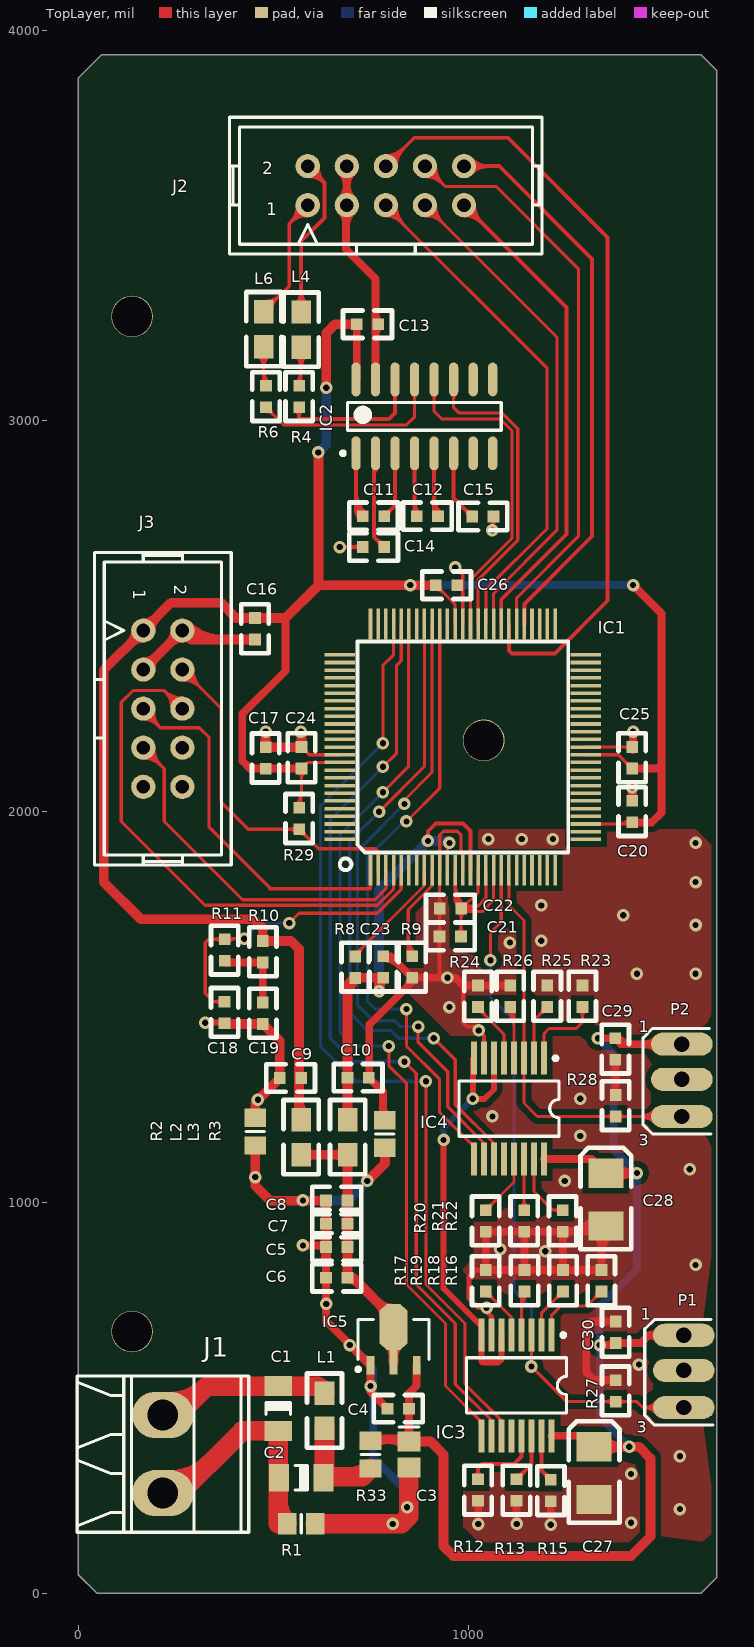
[diagram p0: TopLayer view]
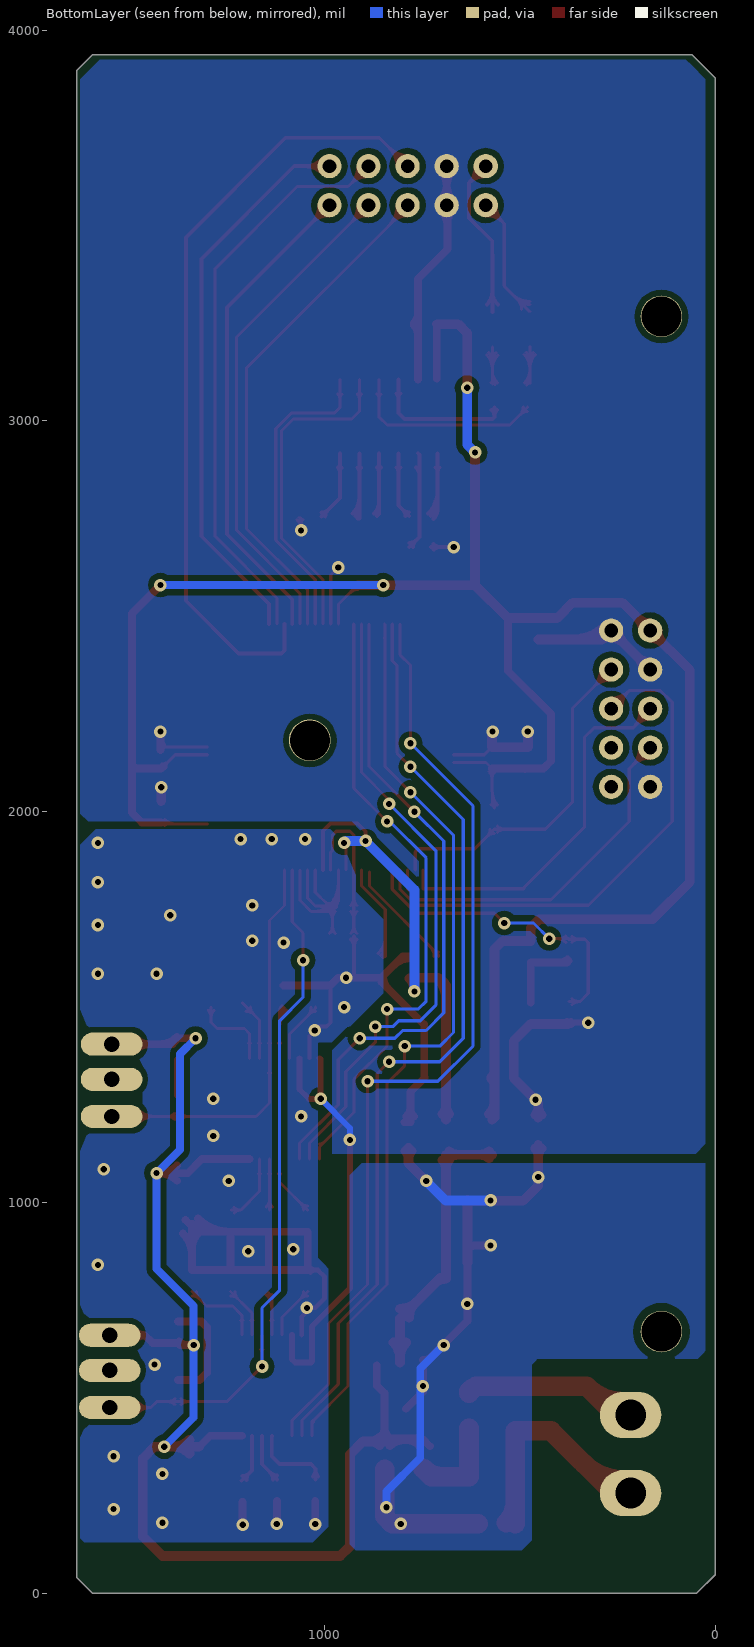
[diagram p1: BottomLayer view, seen from below]
# Altium PCB MISC67359.PcbDoc
Units mil, origin at the board's own origin, x right, y up, seen from the top; angles counter-clockwise.
Board outline 1633.86 x 3937.01 mil, 2 copper layers (TopLayer, BottomLayer); 72 components, 87 nets, 307 pads, 79 vias.

## Layer stack, top to bottom (the 12.6 mil dielectric is the usual default, probably not edited)
TopLayer: signal copper 1.4
Dielectric: core 12.6, FR-4, Dk 4.8
BottomLayer: signal copper 1.4

## Board outline
47.25,0 0,47.24 0,3877.95 59.06,3937.01 1594.49,3937.01 1633.86,3897.64 1633.86,39.37 1594.49,0

## Design rules (kind name [scope] priority, off if disabled: settings)
Clearance Clearance_1 [All vs InNet('DGND_MCU')] p1: gap=15
Clearance [All] p2: gap=8
DiffPairsRouting [All] p1: maxlimit=7 minlimit=7 mostfreqgap=7 maxuncoupledlength=500
FabricationTestPointUsage TestPointUsage [All] p1: valid=0 allowmultiple=FALSE
FabricationTestpoint Testpoint [All] p1: side=3 testpointundercomponent=TRUE minsize=40 maxsize=100 preferedsize=60 minholesize=20 maxholesize=40 preferedholesize=32 testpointgrid=1 allowsidetop=TRUE allowsidebottom=TRUE usegrid=TRUE gridtolerance=0.01
PlaneClearance [All] p1: clearance=10
PlaneConnect [All] p1: planeconnectstyle=Direct reliefexpansion=20 reliefentries=4 reliefconductorwidth=10 reliefairgap=10
PolygonConnect [All] p1: connectstyle=Direct reliefconductorwidth=12 reliefentries=4 polygonreliefangle="90 Angle"
RoutingLayers [All] p1: top layer_v5=FALSE bottom layer_v5=FALSE
RoutingVias [All] p1: holewidth=10 width=20 viastyle="Through Hole" minholewidth=10 minwidth=20 maxholewidth=28 maxwidth=50
SilkscreenOverComponentPads [All] p1: minsilkscreentomaskgap=10
SolderMaskExpansion [All] p1: expansion=4
Width width [All] p1: maxlimit=200 minlimit=7 preferedwidth=8
21 further rules are at their usual default settings.

## Components (designator, comment, footprint, x,y, rotation, side; value= is the part's Value field where it differs from the comment)
C1 "" CAPC3216N 511.81,472.44 r270 top (schematic designator C158)
C2 "" CAPC3216N 570.87,295.28 r180 top (schematic designator C158)
C3 "10u" CAPC2012N 846.46,354.33 r270 top (schematic designator C158)
C4 "0.1U" 0603 846.46,472.44 r180 top (schematic designator C158)
C5 "100n/50V" 0603 688.87,886.23 r180 top (schematic designator C158)
C6 "10n/50V" 0603 688.87,807.49 r180 top (schematic designator C158)
C7 "0.1U" 0603 634.08,945.28 r0 top (schematic designator C158)
C8 "0.1U" 0603 634.08,1004.34 r0 top (schematic designator C158)
C9 "0.1U" 0603 570.87,1318.9 r180 top (schematic designator C158)
C10 "0.1U" 0603 688.98,1318.9 r0 top (schematic designator C158)
C11 "100n/50V" 0603 728.35,2755.91 r0 top (schematic designator C158)
C12 "100n/50V" 0603 866.14,2755.91 r0 top (schematic designator C158)
C13 "100n/50V" 0603 767.72,3248.03 r180 top (schematic designator C158)
C14 "100n/50V" 0603 728.35,2677.17 r0 top (schematic designator C158)
C15 "100n/50V" 0603 1062.99,2755.91 r180 top (schematic designator C158)
C16 "0.1U" 0603 452.76,2440.94 r90 top (schematic designator C158)
C17 "0.1U" 0603 480,2110 r90 top (schematic designator C158)
C18 "1U" 0603 375.01,1458.85 r90 top (schematic designator C158)
C19 "0.1U" 0603 472.84,1456.8 r90 top (schematic designator C158)
C20 "0.1U" 0603 1417.32,2027.56 r270 top (schematic designator C158)
C21 "0.1U" 0603 925,1680 r0 top (schematic designator C158)
C22 "4.7U" 0603 925.2,1751.97 r0 top (schematic designator C158)
C23 "0.1U" 0603 780.2,1629.8 r270 top (schematic designator C158)
C24 "0.1U" 0603 570.87,2165.35 r270 top (schematic designator C158)
C25 "0.1U" 0603 1417.32,2165.35 r270 top (schematic designator C158)
C26 "0.1U" 0603 970,2580 r180 top (schematic designator C158)
C27 "22u" 3528 1320,375 r90 top
C28 "22u" 3528 1350,1075 r90 top
C29 "1U" 0603 1375,1365 r90 top (schematic designator C158)
C30 "1U" 0603 1375,695 r270 top (schematic designator C158)
IC1 "C8051F040" TQFP100 984.25,2165.35 r0 top
IC2 "MAX3232" SOIC127P600-16N 885.83,3011.81 r90 top (schematic designator J2)
IC3 "74HC-HCT4051" SOIC16 1122.05,531.5 r180 top
IC4 "74HC-HCT4051" SOIC16 1102.36,1240.16 r180 top
IC5 "AS117" SOT89L 807.09,649.61 r90 top
J1 "" MKDS3_2RMI 216.54,255.91 r90 top
J2 "" FKV10SN 787.4,3602.36 r0 top
J3 "" FKV10SN 216.54,2263.78 r270 top
L1 "1UH" 0805 629.92,511.81 r270 top (schematic designator C3)
L2 "1UH" 0805 570.87,1122.05 r90 top (schematic designator C3)
L3 "1UH" 0805 688.98,1211.84 r270 top (schematic designator C3)
L4 "600Ω/500mA-0805" 0805 570.87,3188.98 r90 top (schematic designator C3)
L6 "600Ω/500mA-0805" 0805 475,3190 r90 top (schematic designator C3)
P1 "" E3 1545,570 r0 top (schematic designator P2)
P2 "" E3 1540,1315 r0 top
R1 "0R" 6-0805_N 570.87,177.17 r0 top
R2 "0R" 6-0805_N 452.76,1181.1 r90 top
R3 "0R" 6-0805_N 785,1175 r90 top
R4 "100" 0603 565,3090 r270 top (schematic designator C158)
R6 "100" 0603 480,3090 r270 top (schematic designator C158)
R8 "0R" 0603 709.06,1574.7 r90 top (schematic designator C158)
R9 "0R" 0603 855,1575 r90 top (schematic designator C158)
R10 "10K" 0603 472.84,1614.28 r90 top (schematic designator C158)
R11 "1K" 0603 375.22,1618.54 r90 top (schematic designator C158)
R12 "10M 1%" 0603 1023.62,236.22 r90 top (schematic designator C158)
R13 "1M 1%" 0603 1122.05,236.22 r90 top (schematic designator C158)
R15 "100k 1%" 0603 1210,235 r90 top (schematic designator C158)
R16 "10k 1%" 0603 1338.58,826.77 r270 top (schematic designator C158)
R17 "1k 1%" 0603 1043.31,771.98 r90 top (schematic designator C158)
R18 "200R 1%" 0603 1240.16,826.77 r270 top (schematic designator C158)
R19 "100R 1%" 0603 1141.73,826.77 r270 top (schematic designator C158)
R20 "10M 1%" 0603 1043.31,925.2 r90 top (schematic designator C158)
R21 "1M 1%" 0603 1141.73,925.2 r90 top (schematic designator C158)
R22 "100k 1%" 0603 1240.16,925.2 r90 top (schematic designator C158)
R23 "10k 1%" 0603 1290,1555 r270 top (schematic designator C158)
R24 "1k 1%" 0603 1023.62,1500.32 r90 top (schematic designator C158)
R25 "200R 1%" 0603 1200,1555 r270 top (schematic designator C158)
R26 "100R 1%" 0603 1105,1555 r270 top (schematic designator C158)
R27 "100M 1%" 0603 1375,545 r270 top (schematic designator C158)
R28 "100M 1%" 0603 1375,1275 r270 top (schematic designator C158)
R29 "4.7K" 0603 565,2010 r270 top (schematic designator C158)
R33 "0R" 6-0805_N 748.03,354.33 r90 top

## Footprints (in the part's own frame and the unit in brackets; to place one, negate y for a bottom-side part, rotate by r counter-clockwise, add the part's x,y. Pads: shape width x height; smd on the part's side, far side on the other; paste and mask are expansions set on the pad)
6-0805_N [mm] "Chip Resistor, Body 2.0x1.2mm, IPC Medium Density"
  rect 1.2x1.4 smd: 1(-0.9,0) 2(0.9,0)
  silkscreen extent 0,-0.6 0,0.6, body extent -1.07,-0.7 1.07,0.7, height 0.7
0603 [mil]
  rect 30x30 smd: 1(-0.1,0.4) 2(54.9,0.4)
  silkscreen extent -35,-35 90,35
0805 [mil]
  rect 60x50 smd: 1(-0.1,0.38) 2(89.9,0.38)
  silkscreen extent -50,-45 140,45
3528 [mil]
  rect 75x90 smd: 1(-0.28,-0.48) 2(-135.28,-0.48)
  silkscreen extent -195,-65 65,65
CAPC2012N [mm] "Chip Capacitor, Body 2.0x1.3mm, IPC Medium Density"
  rect 1.3x1.5 smd: 1(-0.85,0) 2(0.85,0)
  silkscreen extent -1.8,-0.65 -1.8,0.65, body extent -1.1,-0.72 1.1,0.72, height 1.1
CAPC3216N [mm] "Chip Capacitor, Body 3.2x1.6mm, IPC Medium Density"
  rect 1.3x1.8 smd: 1(-1.45,0) 2(1.45,0)
  silkscreen extent -0.4,-0.8 0.4,0.8, body extent -1.7,-0.9 1.7,0.9, height 1.35
E3 [mm] "TO, Flat Index; 3 In-Line, Axial Leads; Body Dia. 4.6mm; Lead Dia. 0.5 mm (max)"
  oval 4x1.5 hole 1: 1(0.127,2.286) 2(0.127,0) 3(0.127,-2.413)
  silkscreen extent -2.41,-3.56 2.03,3.3
FKV10SN [mil]
  round 62 hole 35: 1(-200,-50) 2(-200,50) 3(-100,-50) 4(-100,50) 5(0,-50) 6(0,50) 7(100,-50) 8(100,50) 9(200,-50) 10(200,50)
  silkscreen extent -400,-175 400,175
MKDS3_2RMI [mm]
  oval 3x4 hole 2: 1(0,0) 2(5.08,0)
  silkscreen extent -2.54,-5.59 7.62,5.59
SOIC16 [mm]
  rect 0.4x2.15 smd: 1(-2.275,-3.275) 2(-1.625,-3.275) 3(-0.975,-3.275) 4(-0.325,-3.275) 5(0.325,-3.275) 6(0.975,-3.275) 7(1.625,-3.275) 8(2.275,-3.275) 9(2.275,3.275) 10(1.625,3.275) 11(0.975,3.275) 12(0.325,3.275) 13(-0.325,3.275) 14(-0.975,3.275) 15(-1.625,3.275) 16(-2.275,3.275)
  silkscreen extent -3.25,-3.4 3.25,1.8
SOIC127P600-16N [mm] "SOIC, 16-Leads, Body 9.9x3.9mm, Pitch 1.27mm, IPC Medium Density"
  oval 2.2x0.6 smd: 1(-2.4,4.445) 2(-2.4,3.175) 3(-2.4,1.905) 4(-2.4,0.635) 5(-2.4,-0.635) 6(-2.4,-1.905) 7(-2.4,-3.175) 8(-2.4,-4.445) 9(2.4,-4.445) 10(2.4,-3.175) 11(2.4,-1.905) 12(2.4,-0.635) 13(2.4,0.635) 14(2.4,1.905) 15(2.4,3.175) 16(2.4,4.445)
  silkscreen extent -2.52,-5 0.9,5.42, body extent -2,-5 2,5, height 1.75
SOT89L [mm] "SOT89, 3-Leads, Body 4.5x2.4 mm, Pitch 1.5mm, Lead Span 4.1mm, IPC High Density"
  rect 1.2x0.5 smd: 1(-1.7,1.5) 3(-1.7,-1.5)
  rect 1.6x0.5 smd: 2(-1.5,0)
  oct 3x1.8 smd: 2(0.8,0)
  silkscreen extent -2.07,-2.3 1.3,2.42, body extent -1.3,-2.3 1.3,2.3, height 1.6
TQFP100 [mm]
  rect 0.23x2 smd: 1(-6,-8) 2(-5.5,-8) 3(-5,-8) 4(-4.5,-8) 5(-4,-8) 6(-3.5,-8) 7(-3,-8) 8(-2.5,-8) 9(-2,-8) 10(-1.5,-8) 11(-1,-8) 12(-0.5,-8) 13(0,-8) 14(0.5,-8) 15(1,-8) 16(1.5,-8) 17(2,-8) 18(2.5,-8) 19(3,-8) 20(3.5,-8) 21(4,-8) 22(4.5,-8) 23(5,-8) 24(5.5,-8) 25(6,-8) 51(6,8) 52(5.5,8) 53(5,8) 54(4.5,8) 55(4,8) 56(3.5,8) 57(3,8) 58(2.5,8) 59(2,8) 60(1.5,8) 61(1,8) 62(0.5,8) 63(0,8) 64(-0.5,8) 65(-1,8) 66(-1.5,8) 67(-2,8) 68(-2.5,8) 69(-3,8) 70(-3.5,8) 71(-4,8) 72(-4.5,8) 73(-5,8) 74(-5.5,8) 75(-6,8)
  rect 2x0.23 smd: 26(8,-6) 27(8,-5.5) 28(8,-5) 29(8,-4.5) 30(8,-4) 31(8,-3.5) 32(8,-3) 33(8,-2.5) 34(8,-2) 35(8,-1.5) 36(8,-1) 37(8,-0.5) 38(8,0) 39(8,0.5) 40(8,1) 41(8,1.5) 42(8,2) 43(8,2.5) 44(8,3) 45(8,3.5) 46(8,4) 47(8,4.5) 48(8,5) 49(8,5.5) 50(8,6) 76(-8,6) 77(-8,5.5) 78(-8,5) 79(-8,4.5) 80(-8,4) 81(-8,3.5) 82(-8,3) 83(-8,2.5) 84(-8,2) 85(-8,1.5) 86(-8,1) 87(-8,0.5) 88(-8,0) 89(-8,-0.5) 90(-8,-1) 91(-8,-1.5) 92(-8,-2) 93(-8,-2.5) 94(-8,-3) 95(-8,-3.5) 96(-8,-4) 97(-8,-4.5) 98(-8,-5) 99(-8,-5.5) 100(-8,-6)
  silkscreen extent -8,-8 6.86,6.86

## Part data
C1 C3: library part Cap2, "Capacitor"
C2: library part CAP, "Capacitor"
C4 C7 C8 C9 C10 C16 C17 C18 C19 C20 C21 C22 C23 C24 C25 C26 C29 C30: library part CAP, "Capacito"
C5 C6 C11 C12 C13 C14 C15: library part "CAPACITOR NON-PO"
C27 C28: library part "CAPACITOR POL"
IC1: library part C8051F020
IC3 IC4: library part CD54HC4051
IC5: library part "Volt Reg", "Voltage Regulator"
J1: library part "Header 2", "Header, 2-Pin"
J2 J3: library part "HEADER 5X2"
L1 L2 L3: library part INDUCTO
L4 L6: library part BEA
P1 P2: library part MHDR1X3
R1 R2 R3 R33: library part RES, "Resistor"
R4 R6: library part SMDRXX_
R8 R9: library part RES, "Resisto"
R10 R11 R12 R13 R15 R16 R17 R18 R19 R20 R21 R22 R23 R24 R25 R26 R27 R28 R29: library part RES

## Free pads (board coordinates)
  round 106.3 hole 102.36: 0(137.8,669.29) 0(137.8,3267.72) 0(1037.8,2182.72)

## Via types
v1: diameter 32, hole 16, TopLayer to BottomLayer, 79 vias

## Nets (pads, with @x,y where several pads share a name; then routed paths per layer and width w, separated by ;. In a path a pad name is that pad's centre, name@x,y a point inside that pad or via, vN(x,y) a via of type N, cw(c..) or ccw(c..) an arc to the next point about the centre after c; other vN are vias at no path point)
3.3VA_MCU: C10.1 C23.2 IC1.11 IC1.14 L3.1 R8.1 | length 1454.6
  TopLayer w8: IC1.11 944.88,1914.88 v1(950,1920)
  TopLayer w10: v1(895,1925) 895,1950 915,1970 985,1970 1003.94,1951.06 IC1.14
  TopLayer w25: L3.1@680.52,1225.78 ccw(c659.18,1247.12) 689.36,1247.12 ccw(c719.54,1247.12) L3.1@698.2,1225.78 ; L3.1 689.36,1555 709.17,1574.8 C23.2@770,1574.8 ; 689.36,1521.96 cw(c761.3,1521.96) R8.1@710.43,1572.83 ; 689.36,1547.09 cw(c715.12,1547.09) R8.1@709.23,1572.16 ; v1@770,1543.28 cw(c812.22,1543.28) C23.2@782.37,1573.14 ; C23.2@770,1574.31 v1(770,1540) v1@770.6,1540.6
  BottomLayer w25: v1@770.6,1540.6 770,1541.2 770,1800 v1(895,1925) 945,1925 v1(950,1920)
3.3VD_MCU: C9.1 C13.2 C16.2 C17.1 C20.2 C24.2 C25.2 C26.2 IC1.28 IC1.37 IC1.64 IC1.90 IC2.16 J3.1 L2.2 R10.2 R29.1 | length 6622.1
  TopLayer w8: C17.1 C24.2@564.6,2109.9 ; C17.1@487.38,2102.12 cw(c506.16,2083.34) 506.16,2109.9 cw(c506.16,2136.45) C17.1@487.38,2117.68 ; 543.36,2109.9 ccw(c543.36,2138.36) C24.2@563.49,2118.23 ; 546.06,2109.9 cw(c546.06,2085.25) 563.49,2102.68 cw(c544.71,2083.9) 571.27,2083.9 cw(c597.82,2083.9) C24.2@579.05,2102.68 ; R29.1@557.62,2017.88 ccw(c527.74,2047.76) 570,2047.76 ; R29.1@563.28,2012.22 ccw(c547.06,2028.45) 570,2028.45 ; R29.1 570,2014.7 570,2050 ; 570,2025.56 ccw(c580.86,2025.56) R29.1@573.18,2017.88 ; 571.27,2051.27 C24.2 586.8,2125.98 IC1.90 ; C26.2@915.1,2568.6 cw(c915.1,2541.32) 934.39,2560.61 ; C26.2 932.55,2562.15 ; C26.2@915.69,2568.61 cw(c916.87,2546.47) 932.55,2562.15 ; C26.2@915.77,2568.62 cw(c917.13,2546.43) 932.85,2562.15 ; C26.2@926.09,2579.01 ccw(c948.23,2577.83) 932.55,2562.15 ; C26.2@926.1,2579.24 ccw(c949.18,2578.48) 932.85,2562.15 ; C26.2@926.1,2579.6 ccw(c951.94,2579.6) 933.67,2561.33 ; IC1.64 964.57,2530.43 932.85,2562.15 ; IC1.28 C20.2@1413.57,1968.5 ; IC1.37 1382.51,2145.67 C25.2 ; 1381.13,1968.5 ccw(c1381.13,2009.25) C20.2@1409.95,1980.44 ; 1400.45,1968.5 ccw(c1400.45,1989.94) C20.2@1415.6,1974.78 ; 1401.2,1968.5 cw(c1401.2,1956.14) C20.2@1409.95,1964.88 ; C25.2@1406.72,2110.46 ccw(c1380.17,2110.46) 1398.95,2129.23 ccw(c1417.72,2148.01) C25.2@1417.72,2121.46 ; 932.55,2562.15 932.85,2562.15
  TopLayer w20: 530.84,2495.84 530.84,2360.84 420,2250 420,2130 439.54,2110.46 C24.2 ; IC2.16@712.82,3108.29 C13.2 ; C20.2 1467.66,1972.66 1492.66,1997.66 1492.66,2120 ; C25.2 1483.12,2110.46 1492.66,2120 ; v1(1420,2580) 1492.66,2507.34 1492.66,2120
  TopLayer w25: J3.1@148.04,2463.78 cw(c103.37,2463.78) 134.95,2432.2 cw(c166.54,2400.62) J3.1@166.54,2445.28 ; J3.1@166.54,2482.28 ccw(c166.54,2526.94) 198.12,2495.36 ccw(c229.7,2463.78) J3.1@185.04,2463.78 ; 565,1260.36 ccw(c613.9,1260.36) L2.2@579.32,1225.78 ; 565,1298.05 cw(c591.41,1298.05) C9.1@572.74,1316.73 ; 565,1338.94 ccw(c591.41,1338.94) C9.1@572.74,1320.26 ; L2.2 565,1217.43 565,1648.35 544.17,1669.17 R10.2 472.44,1702.56 450,1725 160,1725 65,1820 65,2362.24 J3.1 237.76,2535 365,2535 404.16,2495.84 C16.2 530.84,2495.84 614.6,2579.6 ; v1(614.6,2919.6) 614.6,2579.6 ; v1(635,3085) 635,3225 657.63,3247.63 C13.2 ; C26.2 614.6,2579.6
  BottomLayer w20: v1(850,2580) v1(1420,2580)
  BottomLayer w25: v1(614.6,2919.6) 635,2940 v1(635,3085)
3V3: C5.1 C6.1 C7.2 C8.2 IC5.2 L2.1 L3.2 | length 1054.1
  TopLayer w25: L2.1 688.59,1121.95 688.98,1121.56 C8.2 C7.2 C5.1 C6.1 702.91,807.09 807.09,702.91 807.09,681.1 IC5.2@807.09,590.55 ; L2.1@579.32,1113.11 cw(c600.66,1091.77) 600.66,1121.95 cw(c600.66,1152.12) L2.1@579.32,1130.78 ; L3.2@680.52,1108.11 cw(c660.1,1087.69) 688.98,1087.69 ; L3.2@680.52,1113.11 ccw(c659.18,1091.77) 659.18,1121.95 ccw(c659.18,1152.12) L3.2@680.52,1130.78 ; C6.1@688.98,804.59 cw(c688.98,764.9) 717.04,792.96 ; 688.98,1085.85 cw(c720.46,1085.85) L3.2@698.2,1108.11 ; 764.85,745.15 ccw(c807.09,787.4) IC5.2@807.09,727.66 ; 769.22,740.78 cw(c733.16,704.72) IC5.2@784.15,704.72 ; IC5.2@790.87,641.26 cw(c751.72,602.12) 807.09,602.12 cw(c862.45,602.12) IC5.2@823.3,641.26
+5V: C3.1 C4.1 C27.1 C28.1 C29.2 C30.2 IC3.16 IC4.16 IC5.3 P1.1 P2.1 R33.2 | length 4106.7
  TopLayer w20: R33.2@730.42,376.09 R33.2@748.03,393.7 ; C3.1@835.43,398.82 ccw(c808.82,425.43) 846.46,425.43 ccw(c884.1,425.43) C3.1@857.48,398.82 ; C3.1@846.46,388.09 846.46,511.81 866.14,531.5 IC5.3 ; IC4.16 1313.98,1111.22 C28.1 1429.72,1074.72 v1(1430,1075) ; IC3.16 1292.64,402.56 C27.1 ; v1(1330,1420) 1374.5,1420 C29.2 1389.5,1405 P2.1 ; v1(1335,635) 1370.3,635 C30.2 1440.1,640.1 1460,660 ; 1351.01,635 ccw(c1351.01,664.49) C30.2@1371.87,643.64 ; C28.1@1377.43,1055.27 cw(c1424.37,1008.32) 1424.37,1074.72 cw(c1424.37,1141.11) C28.1@1377.43,1094.16 ; C29.2@1378.13,1423.43 ccw(c1422.64,1467.93) 1422.64,1405 ; P2.1@1481.98,1391.19 ccw(c1448.64,1357.86) 1448.64,1405 ccw(c1448.64,1452.14) P2.1@1481.98,1418.81 ; P1.1@1485.58,647.76 ccw(c1460,627.17) 1460,660 ; P1.1@1485.58,672.24 cw(c1460,692.83) 1460,660 ; P1.1 1460,660
  TopLayer w25: R33.2@759.83,381.9 cw(c788.32,353.41) 788.32,393.7 ; R33.2@767.72,393.7 C3.1@828.94,393.7 ; 796.66,393.7 cw(c796.66,341.93) C3.1@833.26,378.54 ; C3.1 902.2,387.8 935,355 935,120 960,95 1415,95 1465,145 1465,345 1435.28,374.72 C27.1 ; C3.1@859.65,378.54 cw(c882,356.19) 882,387.8 cw(c882,419.4) C3.1@859.65,397.05 ; C27.1@1345.66,357.04 cw(c1388.34,314.36) 1388.34,374.72 cw(c1388.34,435.07) C27.1@1345.66,392.39
  BottomLayer w20: v1(1330,1420) 1370,1380 1370,1135 v1(1430,1075) 1430,830 1335,735 v1(1335,635) 1335,449.72 v1(1410,374.72)
/RD: IC1.92
/WR: IC1.91
A0: IC1.80
A1: IC1.79
A1N0.0: IC1.18 IC3.3 P1.3 R27.2 | length 2077.4
  TopLayer w8: v1(1055,1620) 1055,1690 1082.68,1717.68 IC1.18 ; IC3.3@1157.69,623.24 cw(c1151.08,616.63) 1160.43,616.63 cw(c1169.79,616.63) IC3.3@1163.17,623.24 ; v1(1160,580) v1@1160.43,579.57 ; IC3.3 v1@1160.43,579.57 ; R27.2@1367.62,482.32 ccw(c1348.84,463.55) 1348.84,490.1 ccw(c1348.84,516.66) R27.2@1367.62,497.88 ; R27.2@1383.18,482.32 cw(c1401.96,463.55) 1401.96,490.1 cw(c1401.96,516.66) R27.2@1383.18,497.88 ; P1.3@1481.47,458.31 ccw(c1445,426.81) 1445,475 ; P1.3@1481.47,491.69 cw(c1445,523.19) 1445,475 ; P1.3@1487.52,463.54 ccw(c1462.48,441.91) 1462.48,475 ccw(c1462.48,508.09) P1.3@1487.52,486.46 ; P1.3 1445,475 ; v1@1160.43,579.57 1249.9,490.1 R27.2 1429.9,490.1 1445,475
  BottomLayer w8: v1(1055,1620) 1055,1525 1115,1465 1115,775 1160,730 v1(1160,580)
A1N0.1: IC1.19 IC4.3 P2.3 R28.2 | length 1306.6
  TopLayer w8: IC1.19 1102.36,1760 1140.75,1721.61 IC4.3 1140.75,1254.25 1175,1220 P2.3 ; IC4.3@1138.01,1331.91 cw(c1131.4,1325.29) 1140.75,1325.29 cw(c1150.1,1325.29) IC4.3@1143.49,1331.91 ; IC4.3@1138.01,1406.28 ccw(c1131.4,1412.9) 1140.75,1412.9 ccw(c1150.1,1412.9) IC4.3@1143.49,1406.28 ; 1348.6,1220 ccw(c1348.6,1246.91) R28.2@1367.62,1227.88 ; 1349.09,1220 cw(c1349.09,1193.79) R28.2@1367.62,1212.32 ; R28.2@1383.18,1212.32 cw(c1401.71,1193.79) 1401.71,1220 ; R28.2@1383.18,1227.88 ccw(c1402.2,1246.91) 1402.2,1220 ; P2.3@1477.74,1201.95 ccw(c1434.16,1158.37) 1434.16,1220 ccw(c1434.16,1281.63) P2.3@1477.74,1238.05 ; P2.3@1483.39,1207.61 ccw(c1453.47,1177.68) 1453.47,1220 ccw(c1453.47,1262.32) P2.3@1483.39,1232.39
A2: IC1.78
A3: IC1.77
A4: IC1.76
A5: IC1.75
A6: IC1.74
A7: IC1.73
A8: IC1.88
A9: IC1.87
A10: IC1.86
A11: IC1.85
A12: IC1.84
A13: IC1.83
AGND_MCU: C10.2 C21.1 C22.1 C23.1 C27.2 C28.2 C29.1 C30.1 IC1.10 IC1.13 IC3.7 IC4.7 R3.2 R9.1 R12.1 R13.1 R15.1 R16.1 R17.2 R18.1 R19.1 R20.1 R21.1 R22.1 R23.1 R24.2 R25.1 R26.1 R27.1 R28.1 | length 3903.8
  TopLayer w8: C21.1@917.12,1688.18 ccw(c897.87,1707.43) 925.09,1707.43 ; C22.1@917.32,1744.59 cw(c898.54,1725.81) 925.09,1725.81 cw(c951.65,1725.81) C22.1@932.87,1744.59 ; C22.1@917.32,1760.15 ccw(c898.54,1778.93) 925.09,1778.93 ccw(c951.65,1778.93) C22.1@932.87,1760.15 ; C21.1@925.09,1693.31 C22.1 925.09,1850.29 IC1.10 925.2,1940.2 935,1950 970,1950 980,1940 980,1900 985,1895 985,1851.14 IC1.13 ; 925.09,1706.48 ccw(c950.98,1706.48) C21.1@932.68,1688.18
  TopLayer w10: C21.1@917.83,1673.33 cw(c900.76,1656.26) 924.9,1656.26 cw(c949.04,1656.26) C21.1@931.97,1673.33 ; 924.9,1575.1 C21.1 ; 985.22,1555.22 985.22,1459.78 995,1450 1015,1450 1038.39,1426.61 IC4.7 ; R12.1 R12.1@1023.62,235.72
  TopLayer w12: R17.2@1036.54,820.51 ccw(c1021.18,805.15) 1021.18,826.87 ccw(c1021.18,848.6) R17.2@1036.54,833.24 ; R17.2 1016.87,826.87 1000,810 1000,754.29 1024.29,730 1035,730 1058.07,706.93 IC3.7
  TopLayer w20: R3.2@771.43,1220.07 ccw(c750.74,1240.75) 780,1240.75 ; 780,1245.89 ccw(c816.52,1245.89) R3.2@790.7,1220.07 ; C23.1@780.6,1624.91 cw(c780.6,1566.98) 821.56,1607.94 ; C23.1 799.59,1629.91 R9.1@854.5,1575 ; R3.2@795.55,1205 780,1205 780,1283.17 C10.2 745,1320.42 745,1455 854.5,1564.5 R9.1@854.5,1575 ; 838.78,1548.78 ccw(c812.66,1574.9) R9.1@849.6,1574.9 ; R9.1 R9.1@854.5,1575 ; v1@1023.62,177.17 R12.1@1023.62,235.72 ; R26.1@1105.28,1555.22 R24.2 985.22,1555.22 965.44,1575 R9.1@854.5,1575 ; v1@1121.65,177.57 R13.1 ; R21.1@1142.13,924.29 R19.1 ; v1(1209.6,175) R15.1@1209.6,233.95 ; R22.1@1240.56,924.29 R18.1 ; R22.1@1241.29,925.09 ccw(c1241.29,1041.4) C28.2@1323.54,959.16 ; 1289.58,925.09 ccw(c1289.58,993.12) C28.2@1337.68,945.02 ; C28.2@1323.54,920.27 cw(c1286.24,882.98) 1338.98,882.98 ; 1338.98,863.67 cw(c1419.02,863.67) C28.2@1362.43,920.27 ; C28.2@1355.48,954.72 C28.2@1338.98,938.22 ; C29.1 1375.4,1364.1 R28.1 ; R27.1 1319.9,545.1 1300,565 1300,680 1315.1,695.1 C30.1 ; R19.1 R18.1 ; R19.1 R17.2 R20.1 R21.1 R22.1 1325.86,925.09 C28.2@1338.98,938.22 ; R18.1 R16.1 C28.2@1338.98,938.22
  other v1: 1024.02,176.76 1122.05,177.17 1415,180 1540,215 1415,305 1540,350 1435,585 1045,730 1580,840 1195,875 1080,880 1245,1055 1565,1085 1285,1170 1060,1220 1285,1265 1025,1440 950,1500 945,1575 1430,1585 1580,1585 1105,1665 1185,1670 1580,1710 1395,1735 1185,1760 1580,1820 1580,1920 1050,1930 1135,1930 1215,1930
D0: IC1.72 IC3.11 | length 2452.7
  TopLayer w8: v1(780,2175) 780,2375 807.09,2402.09 IC1.72 ; v1(890,1310) 890,790 990,690 990,535 1083.66,441.34 IC3.11
  BottomLayer w8: v1(780,2175) 620,2015 620,1400 710,1310 v1(890,1310)
D1: IC1.71 IC3.10 | length 2400.3
  TopLayer w8: v1(780,2115) 815,2150 815,2375 826.77,2386.77 IC1.71 ; v1(835,1360) 865,1330 865,790 965,690 965,535 1058.07,441.93 IC3.10
  BottomLayer w8: v1(780,2115) 645,1980 645,1420 705,1360 v1(835,1360)
D2: IC1.70 IC3.9 | length 2373.3
  TopLayer w8: v1(780,2050) 845,2115 845,2478.86 IC1.70 ; v1(795,1400) 795,1350 840,1305 840,790 940,690 940,530 1032.48,437.52 IC3.9 ; 845,2440.68 cw(c851.25,2440.68) IC1.70@846.83,2445.1 ; IC3.9@1025.5,444.5 cw(c1018.02,437.01) IC3.9@1028.61,437.01 ; IC3.9@1026.74,443.26 ccw(c1032.48,449) IC3.9@1032.48,440.88
  BottomLayer w8: v1(780,2050) 670,1940 670,1435 705,1400 v1(795,1400)
D3: IC1.69
D4: IC1.68 IC4.11 | length 1688.8
  TopLayer w8: v1(770,2000) 885.83,2115.83 IC1.68 ; v1(910,1420) 965,1365 965,1250 1063.98,1151.02 IC4.11
  BottomLayer w8: v1(770,2000) 695,1925 695,1485 740,1440 800,1440 820,1420 v1(910,1420)
D5: IC1.67 IC4.10 | length 1640.5
  TopLayer w8: v1(835,2020) 835,2030 905.51,2100.51 IC1.67 ; v1(870,1450) 870,1410 945.59,1334.41 945.59,1244.41 1038.39,1151.61 IC4.10
  BottomLayer w8: v1(835,2020) 715,1900 715,1505 755,1465 810,1465 825,1450 v1(870,1450)
D6: IC1.66 IC4.9 | length 1633.6
  TopLayer w8: v1(840,1495) 840,1400 925,1315 925,1230 1012.8,1142.2 IC4.9 ; v1(840,1975) 925.2,2060.2 IC1.66 ; 1000.27,1154.73 ccw(c1012.8,1167.26) IC4.9@1012.8,1149.54
  BottomLayer w8: v1(840,1975) 833.18,1975 740,1881.82 740,1515 760,1495 v1@850,1495
D7: IC1.65
DAC0: IC1.100
DGND_MCU: C9.2 C13.1 C14.1 C15.1 C16.1 C17.2 C18.1 C19.1 C20.1 C24.1 C25.1 C26.1 IC1.38 IC1.63 IC1.89 IC2.15 IC3.6 IC3.8 IC4.6 IC4.8 J2.3 J2.4 J3.2 J3.3 J3.9 R2.2 | length 4031.4
  TopLayer w8: C24.1 591.05,2145.67 IC1.89 ; J2.3@685,3549.96 J2.3 ; v1(965,2625) 984.25,2605.75 IC1.63 ; C15.1@1055.32,2747.73 cw(c1044.01,2736.42) 1060,2736.42 ; v1@1060,2710 v1(1060,2720) C15.1@1060,2751.4 ; v1@1060,2721.48 cw(c1097.12,2721.48) C15.1@1070.87,2747.73 ; C15.1@1060,2740.79 cw(c1077.81,2740.79) C15.1@1065.22,2753.38 ; IC1.38 C25.1@1417.62,2165.35
  TopLayer w10: v1@669.29,2677.57 C14.1 ; C14.1@721.17,2670.5 ccw(c704.1,2653.42) 704.1,2677.57 ccw(c704.1,2701.71) C14.1@721.17,2684.64
  TopLayer w15: v1(325,1460) 396.69,1460 ; 353.48,1460 cw(c353.48,1437.62) C18.1@369.3,1453.44 ; 359.52,1460 ccw(c359.52,1473.83) C18.1@369.3,1464.05 ; C18.1@379.91,1453.44 cw(c395.73,1437.62) 395.73,1460 ; C18.1@379.91,1464.05 ccw(c389.69,1473.83) 389.69,1460 ; v1(935,1160) 935,780 1032.48,682.52 IC3.8 1032.48,592.52 1035,590 1075,590 1083.66,598.66 IC3.6 ; IC4.8 1010,1366.3 v1(1010,1265) 1040,1265 1063.98,1288.98 IC4.6
  TopLayer w20: J2.3@672.55,3537.51 cw(c642.5,3507.46) 685,3507.46 ; J2.3@672.55,3567.21 ccw(c636.7,3603.06) 687.4,3603.06 ccw(c738.1,3603.06) J2.3@702.25,3567.21 ; J2.4@672.55,3637.51 cw(c636.7,3601.66) 687.4,3601.66 cw(c738.1,3601.66) J2.4@702.25,3637.51 ; 685,3495.87 cw(c743.9,3495.87) J2.3@702.25,3537.51 ; J2.3@685,3549.96 685,3440 760.83,3364.17 IC2.15 ; J2.3 J2.4 ; 760.83,3218.68 cw(c796.77,3218.68) C13.1@771.35,3244.09 ; 760.83,3276.58 ccw(c796.77,3276.58) C13.1@771.35,3251.17 ; C25.1@1414.19,2168.99 ccw(c1400.16,2183.02) 1420,2183.02 ; C25.1@1420,2158.18 v1(1420,2205)
  TopLayer w25: J3.3 J3.2 289.47,2440.84 ; J3.3@166.54,2382.28 ccw(c166.54,2426.94) 198.12,2395.36 ccw(c229.7,2363.78) J3.3@185.04,2363.78 ; J3.2@248.04,2463.78 cw(c203.37,2463.78) 234.95,2432.2 cw(c266.54,2400.62) J3.2@266.54,2445.28 ; J3.2@261.94,2459.18 ccw(c306.22,2503.46) 306.22,2440.84 ; J3.2@271.13,2445.86 cw(c275.9,2427.28) 289.47,2440.84 ; J3.2@279.62,2476.86 ccw(c366.57,2563.82) 366.57,2440.84 ; J3.2@284.45,2459.18 ccw(c303.04,2454.41) 289.47,2440.84 ; C18.1 376.66,1456.69 C19.1 515.97,1413.17 C9.2 v1(460,1262.53) 452.76,1255.28 R2.2 ; R2.2@444.89,1224.4 ccw(c425.9,1243.39) 452.76,1243.39 ccw(c479.61,1243.39) R2.2@460.62,1224.4 ; C16.1 289.47,2440.84 ; v1@479.6,2194.6 C17.2 C24.1@570.71,2164.9 ; C24.1 v1@571.27,2196.27 ; C20.1 v1(1417.72,2062.72)
  BottomLayer w8: v1@955,2625 v1(965,2625)
  BottomLayer w15: v1(935,1160) 935,1190 v1(1010,1265)
  other v1: 480,2205 570,2205 669.29,2677.17
GND: C3.2 C4.2 C5.2 C6.2 C7.1 C8.1 IC5.1 R1.2 R2.1 R3.1 | length 2224.4
  TopLayer w20: v1(575,890) 629.8,890 C5.2 ; 611.83,890 cw(c611.83,863.68) C5.2@630.44,882.29 ; 633.98,845 C6.2 633.98,696.73 IC5.1 v1(748.03,530) 748.03,515.57 C4.2 ; 724.78,605.93 ccw(c748.03,629.19) IC5.1@748.03,596.3
  TopLayer w25: R2.1@444.89,1137.8 cw(c425.9,1118.82) 452.76,1118.82 cw(c479.61,1118.82) R2.1@460.62,1137.8 ; R2.1@452.76,1146.59 v1(452.76,1065) 452.76,1043.31 492.13,1003.94 C8.1@633.98,1003.94 ; 633.98,845 C5.2 C7.1 C8.1@633.98,1003.94 ; C8.1 C8.1@633.98,1003.94 ; C8.1@634.78,1003.94 C8.1@633.98,1003.94 ; v1(740,1055) 785,1100 R3.1 ; R3.1@777.14,1131.7 cw(c758.15,1112.72) 785,1112.72 cw(c811.85,1112.72) R3.1@792.86,1131.7
  TopLayer w50: R1.2 v1(805,177.17) 826.77,177.17 846.46,196.85 C3.2@846.46,317.2
  BottomLayer w20: v1(695,635) 755,575 755,346.46 841.46,260 v1(841.46,220)
  BottomLayer w25: v1(575,1005) 690,1005 v1(740,1055)
  other v1: 635,740
HARD_RESET: IC1.53
NetC1_1: C1.1 J1.2 L1.1 | length 587.3
  TopLayer w50: J1.2 255.91,455.91 329.53,529.53 C1.1 612.69,529.53 L1.1 ; J1.2@236.22,489.96 ccw(c236.22,619.7) 327.96,527.96 ; 599.85,529.53 cw(c599.85,486.46) L1.1@630.3,516.91
NetC1_2: C1.2 C2.2 J1.1 R1.1 | length 805
  TopLayer w20: R1.1@511.81,200.79 R1.1
  TopLayer w50: J1.1 260.91,255.91 420.35,415.35 C1.2 511.81,200.79 R1.1@511.81,177.17 ; J1.1@236.22,289.96 ccw(c236.22,431.77) 336.5,331.5 ; 511.81,234.8 ccw(c589.14,234.8) R1.1@534.46,180.13
NetC2_1: C2.1 L1.2 R33.1 | length 305.3
  TopLayer w50: L1.2 630.3,297.63 726.76,297.63 R33.1 ; 696.07,297.63 ccw(c696.07,366.93) R33.1@745.07,317.92
NetC11_1: C11.1 IC2.1 | length 372.1
  TopLayer w10: IC2.1@706.01,2881.01 cw(c694.38,2869.38) 710.83,2869.38 cw(c727.27,2869.38) IC2.1@715.64,2881.01 ; 710.83,2774.21 ccw(c746.15,2774.21) C11.1@721.17,2749.24 ; 710.83,2798.36 ccw(c770.29,2798.36) C11.1 710.83,2773.72 IC2.1 ; 710.83,2822.5 ccw(c794.44,2822.5) C11.1@735.32,2763.38 ; C11.1@718.24,2756.31 ccw(c694.1,2756.31) 711.17,2773.38 ccw(c728.24,2790.45) C11.1@728.24,2766.31
NetC11_2: C11.2 IC2.3 | length 236.2
  TopLayer w10: C11.2 810.83,2783.89 IC2.3 ; C11.2@783.24,2766.31 ccw(c783.24,2790.45) 800.32,2773.38 ccw(c817.39,2756.31) C11.2@793.24,2756.31 ; IC2.3@806.01,2881.01 cw(c794.38,2869.38) 810.83,2869.38 cw(c827.27,2869.38) IC2.3@815.64,2881.01
NetC12_1: C12.1 IC2.4 | length 221.9
  TopLayer w10: IC2.4@856.01,2881.01 cw(c844.38,2869.38) 860.83,2869.38 cw(c877.27,2869.38) IC2.4@865.64,2881.01 ; 860.83,2793.03 ccw(c902.77,2793.03) C12.1@873.11,2763.38 ; IC2.4 860.83,2761.52 C12.1
NetC12_2: C12.2 IC2.5 | length 270.8
  TopLayer w10: IC2.5@906.01,2881.01 cw(c894.38,2869.38) 910.83,2869.38 cw(c927.27,2869.38) IC2.5@915.64,2881.01 ; 910.83,2780.96 ccw(c945.69,2780.96) C12.2 ; 910.83,2805.1 ccw(c969.84,2805.1) C12.2@928.11,2763.38 ; IC2.5 910.83,2750.59 C12.2@915.32,2750.59
NetC14_2: C14.2 IC2.2 | length 312.5
  TopLayer w10: 757.24,2860.73 cw(c785.92,2860.73) IC2.2@765.64,2881.01 ; IC2.2 757.24,2913.74 757.24,2703.57 C14.2 ; C14.2@773.24,2677.57 ccw(c749.1,2677.57) 766.17,2694.64 ccw(c783.24,2711.71) C14.2@783.24,2687.57
NetC15_2: C15.2 IC2.6 | length 245.1
  TopLayer w10: IC2.6@956.01,2881.01 cw(c944.38,2869.38) 960.83,2869.38 cw(c977.27,2869.38) IC2.6@965.64,2881.01 ; IC2.6 960.83,2802.77 C15.2 ; C15.2@998.09,2755.5 ccw(c973.95,2755.5) 991.02,2772.58 ccw(c1008.09,2789.65) C15.2@1008.09,2765.5
NetC18_2: C18.2 IC1.5 R11.2 | length 920.6
  TopLayer w8: C18.2@366.83,1505.97 ccw(c348.05,1487.19) 348.05,1513.75 ccw(c348.05,1540.3) C18.2@366.83,1521.53 ; R11.2@367.04,1665.66 ccw(c348.26,1646.88) 348.26,1673.43 ccw(c348.26,1699.99) R11.2@367.04,1681.21 ; C18.2 346.25,1513.75 325,1535 325,1665 333.43,1673.43 R11.2 376.38,1675 v1(425,1675) ; R11.2@382.6,1665.66 cw(c405.16,1643.09) 405.16,1675 ; R11.2@382.6,1681.21 ccw(c397.59,1696.21) 397.59,1675 ; v1(540,1715) 565,1740 765,1740 826.77,1801.77 IC1.5
  BottomLayer w8: v1(425,1675) 465,1715 v1(540,1715)
NetC19_2: C19.2 R10.1 R11.1 | length 222.8
  TopLayer w20: R11.1 379.08,1614.17 R10.1 C19.2 ; R11.1@378.35,1621.97 ccw(c397.17,1640.79) 397.17,1614.17
NetIC1_1: IC1.1 J3.5 | length 1141.7
  TopLayer w8: J3.5@166.54,2236.78 cw(c166.54,2184.43) 203.55,2221.45 ; J3.5@166.54,2244.78 cw(c166.54,2211.74) 189.9,2235.1 ; J3.5 166.54,2258.46 210,2215 ; J3.5@177.48,2262.73 ccw(c206.91,2259.89) 186.01,2238.99 ; J3.5@185.45,2261.96 ccw(c228.79,2257.79) 198,2227 ; J3.5@193.41,2261.19 ccw(c250.68,2255.68) 210,2215 ; IC1.1 748.03,1802.64 490,1802.64 490,1805 335,1960 335,2190 310,2215 210,2215
NetIC1_2: IC1.2 J3.4 R29.2 | length 1139.9
  TopLayer w8: J3.4@266.54,2336.78 cw(c266.54,2271.6) 312.63,2317.69 cw(c358.72,2363.78) J3.4@293.54,2363.78 ; J3.4@266.54,2344.78 cw(c266.54,2298.91) 298.97,2331.34 cw(c331.41,2363.78) J3.4@285.54,2363.78 ; J3.4 365,2265.31 365,2025 434.9,1955.1 R29.2 615.5,1905 760,1905 767.72,1897.28 IC1.2 ; R29.2@557.62,1947.32 ccw(c538.84,1928.55) 538.84,1955.1 ccw(c538.84,1981.66) R29.2@557.62,1962.88 ; R29.2@565.4,1944.1 cw(c565.4,1917.55) 584.18,1936.32 cw(c602.96,1955.1) R29.2@576.4,1955.1
NetIC1_3: IC1.3 J3.7 | length 1095.2
  TopLayer w8: J3.7@166.54,2136.78 cw(c166.54,2071.6) 212.63,2117.69 cw(c258.72,2163.78) J3.7@193.54,2163.78 ; J3.7@166.54,2144.78 cw(c166.54,2098.91) 198.97,2131.34 cw(c231.41,2163.78) J3.7@185.54,2163.78 ; J3.7 220,2110.31 220,1975 420.36,1774.64 759.63,1774.64 787.4,1802.41 IC1.3
NetIC1_4: IC1.4 J3.6 | length 1518.8
  TopLayer w8: J3.6@239.54,2263.78 ccw(c174.35,2263.78) 220.44,2309.87 ccw(c266.54,2355.96) J3.6@266.54,2290.78 ; J3.6@247.54,2263.78 ccw(c201.67,2263.78) 234.1,2296.21 ccw(c266.54,2328.65) J3.6@266.54,2282.78 ; J3.6 220.31,2310 140,2310 110,2280 110,1975 324.36,1760.64 765.43,1760.64 807.09,1802.3 IC1.4
NetIC1_8: IC1.8 R8.2 | length 330.4
  TopLayer w8: R8.2 708.66,1633.66 885,1810 IC1.8@885,1845.24 ; R8.2@708.66,1640.6 ccw(c708.66,1657.35) 720.5,1645.5 ; R8.2@719.66,1629.6 cw(c756.03,1629.6) 730.31,1655.31
NetIC1_9: IC1.9 R9.2 | length 343.2
  TopLayer w8: R9.2@844.6,1629.9 844.6,1749.6 905.51,1810.51 IC1.9 ; R9.2@844.6,1641.97 ccw(c866.67,1641.97) R9.2@851.06,1626.36 ; 844.6,1661.28 ccw(c885.98,1661.28) R9.2@856.72,1632.02 ; 844.6,1680.6 ccw(c905.3,1680.6) R9.2@862.38,1637.68
NetIC2_13: IC2.13 R6.2 | length 574.5
  TopLayer w8: R6.2@480.4,3024.1 cw(c480.4,2997.55) 499.18,3016.32 cw(c517.96,3035.1) R6.2@491.4,3035.1 ; R6.2 525.5,2990 840,2990 860.83,3010.83 IC2.13 ; IC2.13@855.3,3069.28 cw(c841.97,3055.95) 860.83,3055.95 cw(c879.68,3055.95) IC2.13@866.35,3069.28
NetIC2_14: IC2.14 R4.2 | length 428.6
  TopLayer w10: R4.2@558.33,3028.03 cw(c541.26,3010.96) 565.4,3010.96 cw(c589.54,3010.96) R4.2@572.47,3028.03 ; R4.2 565.4,3009.6 570,3005 795,3005 810.83,3020.83 IC2.14 ; IC2.14@806.01,3069.99 cw(c794.38,3058.36) 810.83,3058.36 cw(c827.27,3058.36) IC2.14@815.64,3069.99
NetIC3_1: IC3.1 R16.2 | length 259.9
  TopLayer w8: IC3.1@1208.87,697.62 ccw(c1202.26,704.23) 1211.61,704.23 ccw(c1220.97,704.23) IC3.1@1214.35,697.62 ; IC3.1 1211.61,711.61 1235,735 1302.11,735 R16.2 ; R16.2@1327.98,771.87 cw(c1301.43,771.87) 1320.21,753.1 cw(c1338.98,734.32) R16.2@1338.98,760.87
NetIC3_2: IC3.2 R18.2 | length 190.4
  TopLayer w8: IC3.2@1183.28,697.62 ccw(c1176.67,704.23) 1186.02,704.23 ccw(c1195.38,704.23) IC3.2@1188.76,697.62 ; IC3.2 1186.02,717.34 R18.2 ; R18.2@1229.56,771.87 cw(c1203,771.87) 1221.78,753.1 cw(c1240.56,734.32) R18.2@1240.56,760.87
NetIC3_4: IC3.4 R19.2 | length 184.5
  TopLayer w8: IC3.4@1132.1,697.62 ccw(c1125.49,704.23) 1134.84,704.23 ccw(c1144.19,704.23) IC3.4@1137.58,697.62 ; IC3.4 R19.2@1134.84,764.58 ; 1134.84,727.71 cw(c1186.29,727.71) R19.2@1149.91,764.1 ; 1134.84,747.03 cw(c1166.98,747.03) R19.2@1144.25,769.75
NetIC3_5: IC3.5 R17.1 | length 180.6
  TopLayer w8: R17.1@1042.91,760.87 cw(c1042.91,734.32) 1061.68,753.1 cw(c1080.46,771.87) R17.1@1053.91,771.87 ; R17.1 1109.25,705.53 IC3.5
NetIC3_13: IC3.13 R12.2 | length 242.6
  TopLayer w10: R12.2@1016.15,298.19 ccw(c999.08,315.26) 1023.22,315.26 ccw(c1047.36,315.26) R12.2@1030.29,298.19 ; R12.2 1023.22,318.22 1035,330 1115,330 1135,350 1135,402.4 IC3.13
NetIC3_14: IC3.14 R13.2 | length 165.4
  TopLayer w10: R13.2 1160.43,329.91 IC3.14 ; R13.2@1121.65,301.12 ccw(c1121.65,325.26) 1138.72,308.19 ccw(c1155.79,291.12) R13.2@1131.65,291.12
NetIC3_15: IC3.15 R15.2 | length 163.9
  TopLayer w10: IC3.15 1186.02,313.98 R15.2@1212.5,287.5 ; 1192.17,307.83 cw(c1174.24,289.9) R15.2@1199.6,289.9 ; 1193.39,306.61 ccw(c1209.6,322.82) R15.2@1209.6,299.9
NetIC4_1: IC4.1 R23.2 | length 269.2
  TopLayer w8: IC4.1@1189.19,1406.28 ccw(c1182.58,1412.9) 1191.93,1412.9 ccw(c1201.28,1412.9) IC4.1@1194.67,1406.28 ; IC4.1 1191.93,1431.93 1205,1445 1275,1445 1290.4,1460.4 R23.2 ; R23.2@1282.62,1492.32 cw(c1263.84,1473.55) 1290.4,1473.55 cw(c1316.96,1473.55) R23.2@1298.18,1492.32
NetIC4_2: IC4.2 R25.2 | length 216.2
  TopLayer w8: IC4.2@1163.6,1406.28 ccw(c1156.99,1412.9) 1166.34,1412.9 ccw(c1175.69,1412.9) IC4.2@1169.08,1406.28 ; IC4.2 1166.34,1466.34 R25.2@1210.55,1510.55 ; 1181.11,1481.11 cw(c1200.4,1461.82) R25.2@1200.4,1489.1 ; 1181.83,1481.83 ccw(c1163.57,1500.1) R25.2@1189.4,1500.1
NetIC4_4: IC4.4 R26.2 | length 245.3
  TopLayer w8: R26.2@1097.62,1492.32 cw(c1055.29,1449.99) 1115.16,1449.99 ; R26.2@1103.28,1497.98 cw(c1074.61,1469.31) 1115.16,1469.31 ; R26.2 1115.16,1490.35 IC4.4 ; R26.2@1108.94,1503.64 cw(c1093.92,1488.62) R26.2@1115.16,1488.62 ; IC4.4@1112.42,1406.28 ccw(c1105.8,1412.9) 1115.16,1412.9 ccw(c1124.51,1412.9) IC4.4@1117.9,1406.28
NetIC4_5: IC4.5 R24.1 | length 200.3
  TopLayer w8: R24.1@1023.22,1489.22 cw(c1023.22,1470.97) 1036.12,1483.88 ; R24.1 1023.22,1496.78 1089.57,1430.43 IC4.5 ; R24.1@1034.22,1500.22 ccw(c1069.09,1500.22) 1044.43,1475.57
NetIC4_13: IC4.13 R20.2 | length 217.5
  TopLayer w8: R20.2 1115.16,1052.35 IC4.13 ; R20.2@1042.91,991.09 ccw(c1042.91,1017.65) 1061.68,998.87 ccw(c1080.46,980.09) R20.2@1053.91,980.09 ; IC4.13@1112.42,1074.03 cw(c1105.8,1067.42) 1115.16,1067.42 cw(c1124.51,1067.42) IC4.13@1117.9,1074.03
NetIC4_14: IC4.14 R21.2 | length 187.8
  TopLayer w8: R21.2@1133.55,987.87 ccw(c1116.18,1005.24) 1140.75,1005.24 ; IC4.14@1138.01,1074.03 cw(c1131.4,1067.42) 1140.75,1067.42 cw(c1150.1,1067.42) IC4.14@1143.49,1074.03 ; 1140.75,1008.06 ccw(c1169.29,1008.06) R21.2@1149.11,987.87 ; IC4.14 1140.75,980.68 R21.2
NetIC4_15: IC4.15 R22.2 | length 228.4
  TopLayer w8: IC4.15@1163.6,1074.03 cw(c1156.99,1067.42) 1166.34,1067.42 cw(c1175.69,1067.42) IC4.15@1169.08,1074.03 ; IC4.15 1166.34,1028.66 1214.91,980.09 ; R22.2@1231.61,972.7 ccw(c1214.91,957.53) 1214.91,980.09 ; R22.2@1231.61,987.49 cw(c1214.91,1002.66) 1214.91,980.09 ; R22.2 1214.91,980.09
NetJ2_1: J2.1 L6.2 | length 607.4
  TopLayer w8: L6.2 540,3345.28 540,3504.96 J2.1 ; L6.2@474.62,3297.9 ccw(c474.62,3341.35) 505.35,3310.63 ; L6.2@474.62,3305.9 ccw(c474.62,3368.67) 519,3324.28 ; L6.2@495.62,3284.9 cw(c534.25,3284.9) 506.93,3312.21 ; J2.1@560.4,3552.36 cw(c495.22,3552.36) 541.31,3506.27 cw(c587.4,3460.18) J2.1@587.4,3525.36 ; J2.1@568.4,3552.36 cw(c522.53,3552.36) 554.97,3519.93 cw(c587.4,3487.49) J2.1@587.4,3533.36
NetJ2_2: J2.2 L4.2 | length 640.6
  TopLayer w10: L4.2@556.34,3298.02 ccw(c522.2,3332.16) 570.48,3332.16 ccw(c618.77,3332.16) L4.2@584.63,3298.02 ; L4.2 570.48,3424.82 570.87,3425.2 570.87,3460.43 629.92,3519.49 629.92,3609.84 ; J2.2 629.92,3609.84 ; J2.2@587.9,3636.37 cw(c588.97,3601.6) 613.57,3626.2 cw(c638.16,3650.8) J2.2@603.39,3651.87 ; J2.2@588.2,3626.37 cw(c589.95,3569.87) 629.92,3609.84 ; J2.2@613.39,3651.56 ccw(c669.89,3649.82) 629.92,3609.84
NetL4_1: L4.1 R4.1 | length 283.7
  TopLayer w8: L4.1@555.64,3169.03 cw(c519.79,3133.18) 570.48,3133.18 cw(c621.18,3133.18) L4.1@585.33,3169.03 ; R4.1@557.62,3097.88 ccw(c526.57,3128.93) 570.48,3128.93 ; L4.1@561.29,3174.68 cw(c539.1,3152.49) 570.48,3152.49 cw(c601.87,3152.49) L4.1@579.68,3174.68 ; R4.1@563.28,3092.22 ccw(c545.89,3109.62) 570.48,3109.62 ; R4.1@570.48,3095.19 L4.1 ; R4.1@570.48,3104.39 ccw(c579.69,3104.39) R4.1@573.18,3097.88
NetL6_1: L6.1 R6.1 | length 280.5
  TopLayer w8: L6.1@459.77,3170.05 cw(c423.92,3134.2) 474.62,3134.2 cw(c525.32,3134.2) L6.1@489.47,3170.05 ; L6.1@465.43,3175.71 cw(c443.23,3153.51) 474.62,3153.51 cw(c506,3153.51) L6.1@483.81,3175.71 ; R6.1@474.62,3095.89 L6.1 ; 474.62,3111.31 ccw(c501.61,3111.31) R6.1@482.52,3092.22 ; 474.62,3130.62 ccw(c520.92,3130.62) R6.1@488.18,3097.88
P0.2: IC1.60 J2.5 | length 1512.2
  TopLayer w8: J2.5@787.4,3525.36 cw(c787.4,3471.68) 825.36,3509.64 ; J2.5@787.4,3533.36 cw(c787.4,3498.99) 811.7,3523.3 ; J2.5 787.4,3547.6 1200,3135 1200,2725 1043.31,2568.31 IC1.60 ; J2.5@798.4,3552.36 ccw(c836.46,3552.36) 809.55,3525.45 ; J2.5@806.4,3552.36 ccw(c863.77,3552.36) 823.21,3511.79 ; J2.5@814.4,3552.36 ccw(c891.09,3552.36) 836.86,3498.14
P0.3: IC1.59 J2.7 | length 1453.6
  TopLayer w8: J2.7@887.4,3525.36 cw(c887.4,3459.61) 933.9,3506.1 ; J2.7@887.4,3533.36 cw(c887.4,3486.92) 920.24,3519.76 ; J2.7 887.64,3552.36 1225,3215 1225,2720 1062.99,2557.99 IC1.59 ; J2.7@906.4,3552.36 ccw(c951.7,3552.36) 919.67,3520.33 ; J2.7@914.4,3552.36 ccw(c979.02,3552.36) 933.33,3506.67
P0.4: IC1.58 J2.9 | length 1409.5
  TopLayer w10: J2.9@987.4,3526.36 cw(c987.4,3463.02) 1032.19,3507.81 ; J2.9@987.4,3536.36 cw(c987.4,3497.16) 1015.12,3524.88 ; J2.9 987.64,3552.36 1250,3290 1250,2710 1082.68,2542.68 IC1.58 ; J2.9@1003.4,3552.36 ccw(c1041.46,3552.36) 1014.55,3525.45 ; J2.9@1013.4,3552.36 ccw(c1075.6,3552.36) 1031.62,3508.38
P0.5: IC1.57 J2.6 | length 2172
  TopLayer w10: J2.6 860.04,3725 1100,3725 1355,3470 1355,2540 1220,2405 1110,2405 1102.36,2412.64 IC1.57 ; J2.6@787.4,3668.36 ccw(c787.4,3706.99) 814.72,3679.68 ccw(c842.03,3652.36) J2.6@803.4,3652.36 ; J2.6@787.4,3678.36 ccw(c787.4,3741.13) 831.79,3696.75 ccw(c876.17,3652.36) J2.6@813.4,3652.36
P0.6: IC1.56 J2.8 | length 1650.8
  TopLayer w8: J2.8@887.4,3625.36 cw(c887.4,3560.18) 933.49,3606.27 cw(c979.59,3652.36) J2.8@914.4,3652.36 ; J2.8@887.4,3633.36 cw(c887.4,3587.49) 919.84,3619.93 cw(c952.27,3652.36) J2.8@906.4,3652.36 ; J2.8 939.76,3600 1070,3600 1280,3390 1280,2705 1122.05,2547.05 IC1.56
P0.7: IC1.55 J2.10 | length 1591.6
  TopLayer w10: J2.10 1077.64,3652.36 1315,3415 1315,2705 1141.73,2531.73 IC1.55 ; J2.10@998.72,3641.05 cw(c1026.03,3613.73) 1026.03,3652.36 cw(c1026.03,3690.99) J2.10@998.72,3663.68 ; J2.10@1005.79,3633.98 cw(c1050.17,3589.59) 1050.17,3652.36 cw(c1050.17,3715.13) J2.10@1005.79,3670.75
P3.6: IC1.48
P3.7: IC1.47
SOFT_RESET: IC1.52
SYS_RESET_L_MCU: IC1.54
UART0_CTS: IC2.9
UART0_RTS: IC2.10
UART0_RXD: IC1.62 IC2.12 | length 869.9
  TopLayer w8: IC2.12@905.3,3069.28 cw(c891.97,3055.95) 910.83,3055.95 cw(c929.68,3055.95) IC2.12@916.35,3069.28 ; IC2.12 910.83,3024.17 930,3005 1080,3005 1110,2975 1110,2700 1003.94,2593.94 IC1.62
UART0_TXD: IC1.61 IC2.11 | length 830
  TopLayer w8: IC2.11@955.3,3069.28 cw(c941.97,3055.95) 960.83,3055.95 cw(c979.68,3055.95) IC2.11@966.35,3069.28 ; IC2.11 960.83,3034.17 975,3020 1085,3020 1125,2980 1125,2695 1023.62,2593.62 IC1.61
VREF: C21.2 C22.2 IC1.12 IC1.15 IC1.16 IC1.17 | length 1026.8
  TopLayer w8: 964.57,1777.79 ccw(c1005.51,1777.79) C22.2@976.56,1748.83 ; 964.57,1797.1 ccw(c1024.82,1797.1) 982.22,1754.49 ccw(c1005.13,1777.4) 1005.13,1745 ; IC1.12@964.57,1816.41 ccw(c1044.14,1816.41) 987.87,1760.15 ccw(c1024.44,1796.72) 1024.44,1745 ; IC1.12 964.57,1770.43 ; 965.65,1769.35 ccw(c980.09,1783.8) 980.09,1763.37 ccw(c980.09,1795.42) 1002.76,1772.76 ; C22.2@969.32,1754.58 ccw(c952.23,1758.1) 964.57,1770.43 ; C21.2@972.12,1688.18 ccw(c952.87,1707.43) 980.09,1707.43 ; C22.2@972.32,1744.59 cw(c953.54,1725.81) 980.09,1725.81 cw(c1006.65,1725.81) 987.87,1744.59 cw(c1021.9,1710.57) 1021.9,1758.68 ; C21.2@980.09,1693.31 C22.2 ; 980.09,1706.48 ccw(c1005.98,1706.48) C21.2@987.68,1688.18 ; C22.2@982.22,1750.25 cw(c1002.58,1729.88) 1002.58,1758.68 ; C22.2@991.09,1752.37 cw(c1012.16,1752.37) 997.26,1767.26 ; IC1.15 1023.62,1793.62 995,1765 C22.2@980.09,1765 ; IC1.16 1043.31,1778.31 1023.68,1758.68 C22.2@980.09,1758.68 ; IC1.17 1062.99,1772.99 1035,1745 987.46,1745 C22.2 ; 964.57,1770.43 970,1765 C22.2@980.09,1765 ; C22.2 C22.2@980.09,1758.68 ; C22.2@980.09,1758.68 C22.2@980.09,1765
pads on no net: IC1.6 IC1.7 IC1.20 IC1.21 IC1.22 IC1.23 IC1.24 IC1.25 IC1.26 IC1.27 IC1.29 IC1.30 IC1.31 IC1.32 IC1.33 IC1.34 IC1.35 IC1.36 IC1.39 IC1.40 IC1.41 IC1.42 IC1.43 IC1.44 IC1.45 IC1.46 IC1.49 IC1.50 IC1.51 IC1.81 IC1.82 IC1.93 IC1.94 IC1.95 IC1.96 IC1.97 IC1.98 IC1.99 IC2.7 IC2.8 IC3.12 IC4.12 J3.8 J3.10 P1.2 P2.2

## Polygon pours and split planes (outlines as drawn)
AGND_MCU on TopLayer "Mechanical 1-No Net" (solid, remove dead copper, pour order 2): 920,1955 915,1950 915,1805 915,1795 890,1770 845,1725 845,1675 845,1535 970,1410 1000,1410 1010,1410 1012.8,1407.2 1012.8,1369.09 1012.8,857.8 995,840 985,830 985,825 985,170 1020,135 1025,130 1285,130 1610,130 1620,140 1620,1870 1620,1915 1580,1955 920,1955 915,1950
GND on BottomLayer "Mechanical 1-No Net" (solid, remove dead copper, pour order 7): 25,1100 905,1100 925,1080 935,1070 935,1040 935,125 920,110 495,110 475,130 470,135 470,170 470,585 460,595 455,600 380,600 45,600 30,615 25,620 25,1100
DGND_MCU on BottomLayer "Mechanical 1-No Net" (solid, remove dead copper, pour order 5): 980,1125 50,1125 25,1150 25,1470 25,3875 60,3910 75,3925 1575,3925 1600,3900 1625,3875 1625,3810 1625,1995 1605,1975 930,1975 880,1925 835,1880 835,1650 835,1535 880,1490 980,1390 980,1125
AGND_MCU on BottomLayer "Mechanical 1-No Net" (solid, remove dead copper, pour order 2): 925,1955 920,1950 920,1805 920,1795 895,1770 850,1725 850,1675 850,1535 975,1410 1005,1410 1015,1410 1017.8,1407.2 1017.8,1369.09 1017.8,857.8 1000,840 990,830 990,825 990,170 1025,135 1030,130 1290,130 1615,130 1625,140 1625,1870 1625,1915 1585,1955 925,1955 920,1950

## Silkscreen, mask and mechanical layers (free items; w line width, h text height)
Mechanical1:
  lines w10: 0,47.24 47.25,0 1594.49,0 1633.86,39.37 1633.86,3307.09 1633.86,3897.64 1594.49,3937.01 59.06,3937.01 0,3877.95 0,47.24